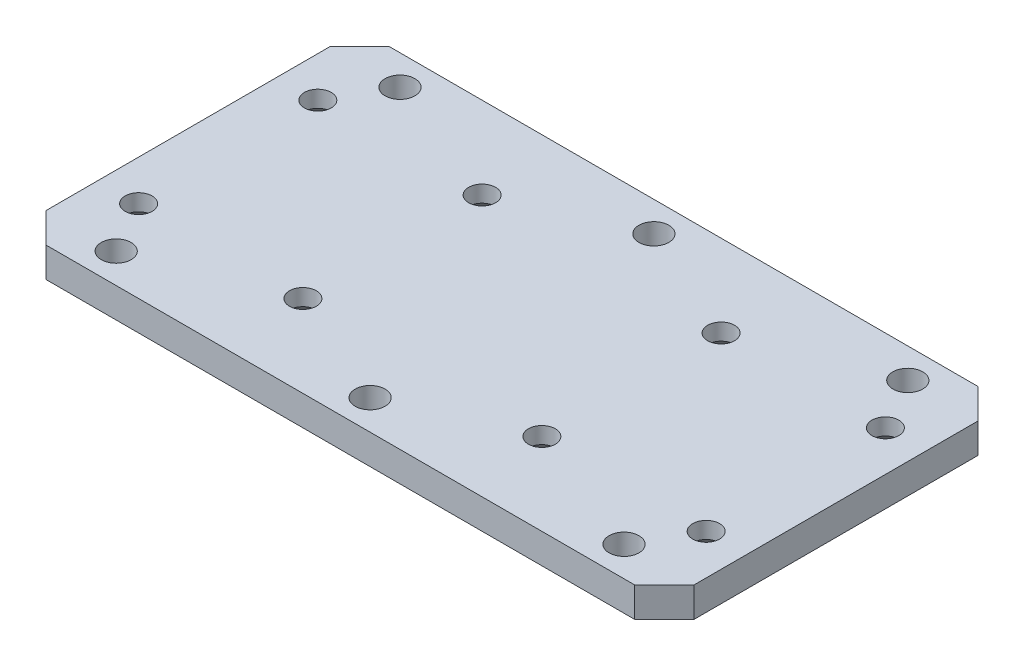
SolidWorks part; units mm, degrees
material "Q235A"
ref_plane "前视基准面" through (0, 0, 0) normal (0, 0, 1) x (1, 0, 0)
ref_plane "上视基准面" through (0, 0, 0) normal (0, 1, 0) x (1, 0, 0)
ref_plane "右视基准面" through (0, 0, 0) normal (1, 0, 0) x (0, 0, -1)
sketch "草图1" plane through (0, 0, 0) normal (0, 1, 0) x (1, 0, 0)
  line L1 (-108.5, -57.5) -> (108.5, -57.5)
  line L2 (-108.5, -57.5) -> (-108.5, 57.5)
  line L3 (-108.5, 57.5) -> (108.5, 57.5)
  line L4 (108.5, -57.5) -> (108.5, 57.5)
  line L5 (-108.5, -57.5) -> (108.5, 57.5) construction
  line L6 (-108.5, 57.5) -> (108.5, -57.5) construction
  point P0 (0, 0)
  dimension "D1" = 115
  dimension "D2" = 217
extrude "凸台-拉伸1" add sketch "草图1" along normal blind 10
hole_wizard "M8 六角凹锥坑螺钉的锥形沉头孔1" positions "草图2" profile "草图3" countersink size "M8" standard "ISO" end condition through all
sketch "草图2" plane through (0, 0, 0) normal (0, -1, 0) x (-1, 0, 0)
  line L0 (0, 0) -> (123.7682, 0) construction
  point P0 (-95, -30)
  point P3 (-40, -30)
  point P6 (40, -30)
  point P9 (95, -30)
  point P17 (95, 30)
  point P18 (40, 30)
  point P19 (-40, 30)
  point P20 (-95, 30)
sketch "草图3" plane through (95, 0, 30) normal (1, 0, 0) x (0, 0, -1)
  line L0 (0, 0) -> (0, 10)
  line L1 (0, 10) -> (4.5, 10)
  line L2 (4.5, 10) -> (4.5, 4.46)
  line L3 (4.5, 4.46) -> (8.96, 0)
  line L5 (8.96, 0) -> (0, 0)
  line L6 (-4.5, 4.46) -> (-8.96, 0) construction
  line L11 (0, -6.35) -> (0, 107.95) construction
  dimension "通孔孔直径" = 9
  dimension "通孔孔深度" = 10
  dimension "近端锥形沉头孔直径" = 17.92
  dimension "近端锥形沉头孔角度" = 90
hole_wizard "M8 间隙孔2" positions "草图4" profile "草图5" hole size "M8" standard "ISO" end condition through all
sketch "草图4" plane through (0, 0, 0) normal (0, -1, 0) x (-1, 0, 0)
  line L0 (0, 57.5) -> (0, 0) construction
  line L1 (-108.5, 57.5) -> (108.5, 57.5) construction
  line L3 (0, 0) -> (133.1203, 0) construction
  point P0 (-85, 47.5)
  point P2 (0, 47.5)
  point P4 (85, 47.5)
  point P17 (85, -47.5)
  point P18 (0, -47.5)
  point P19 (-85, -47.5)
  dimension "D1" = 170
  dimension "D2" = 10
sketch "草图5" plane through (85, 0, -47.5) normal (1, 0, 0) x (0, 0, -1)
  line L0 (0, 0) -> (0, 10)
  line L1 (0, 10) -> (5, 10)
  line L2 (5, 10) -> (5, 0)
  line L5 (5, 0) -> (0, 0)
  line L11 (0, -6.35) -> (0, 107.95) construction
  dimension "通孔孔直径" = 10
  dimension "通孔孔深度" = 10
chamfer "倒角1" distance 10 angle 45 4 edges at (108.5, 5, 57.5) (-108.5, 5, 57.5) (-108.5, 5, -57.5) (108.5, 5, -57.5)
